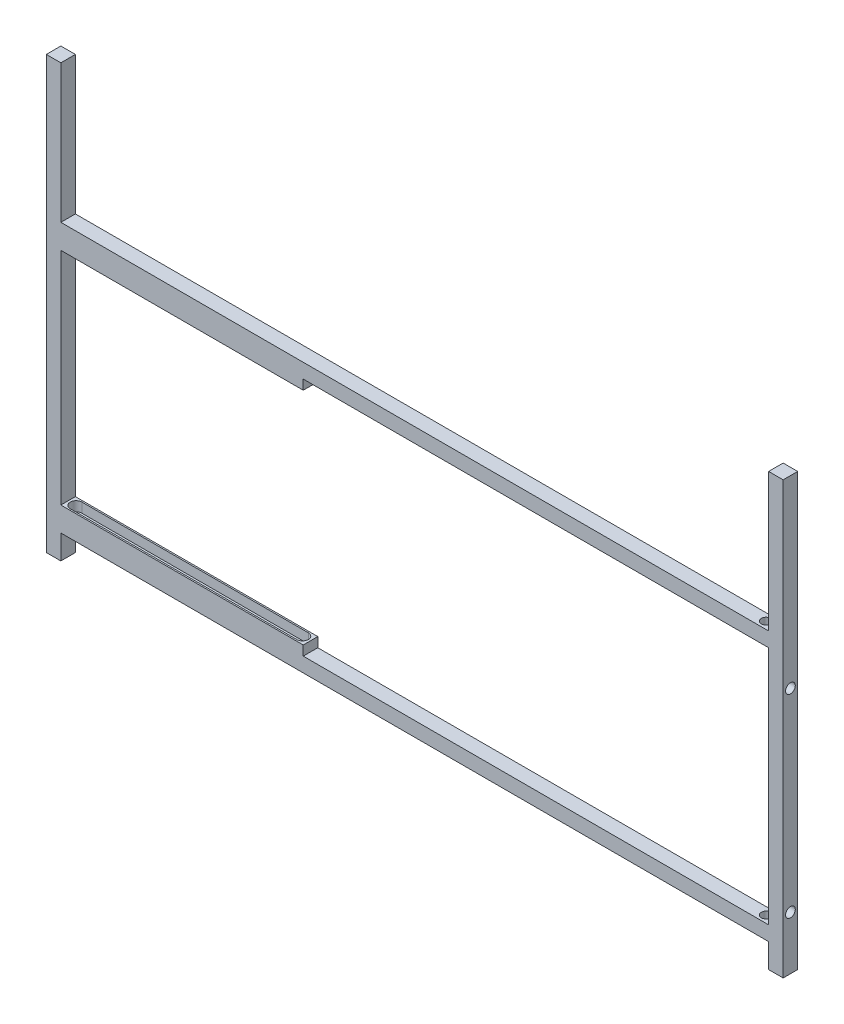
SolidWorks part; units mm, degrees
ref_plane "Front Plane" through (0, 0, 0) normal (0, 0, 1) x (1, 0, 0)
ref_plane "Top Plane" through (0, 0, 0) normal (0, 1, 0) x (1, 0, 0)
ref_plane "Right Plane" through (0, 0, 0) normal (1, 0, 0) x (0, 0, -1)
other "Configuration Table"
sketch "Sketch1" plane through (0, 0, 0) normal (0, 1, 0) x (1, 0, 0)
  line L8 (0, 0) -> (0, 55.1158) construction
  line L9 (-7.5, 7.5) -> (7.5, 7.5)
  line L10 (-7.5, 7.5) -> (-7.5, -7.5)
  line L11 (-7.5, -7.5) -> (7.5, -7.5)
  line L12 (7.5, 7.5) -> (7.5, -7.5)
  line L13 (-7.5, 7.5) -> (7.5, -7.5) construction
  line L14 (-7.5, -7.5) -> (7.5, 7.5) construction
  line L15 (372.5, 47.674) -> (372.5, -59.4029) construction
  line L16 (752.5, -7.5) -> (737.5, -7.5)
  line L17 (737.5, 7.5) -> (737.5, -7.5)
  line L18 (752.5, 7.5) -> (737.5, 7.5)
  line L19 (752.5, 7.5) -> (752.5, -7.5)
  point P0 (0, 0)
  dimension "D1" = 15
  dimension "D2" = 15
  dimension "D3" = 372.5
extrude "Boss-Extrude1" add sketch "Sketch1" against normal blind 445
sketch "Sketch2" plane through (7.5, 0, 0) normal (1, 0, 0) x (0, 0, -1)
  line L0 (7.5, -445) -> (7.5, 0) construction
  line L1 (-7.5, -405) -> (7.5, -405)
  line L2 (-7.5, -405) -> (-7.5, -420)
  line L3 (-7.5, -420) -> (7.5, -420)
  line L4 (7.5, -405) -> (7.5, -420)
  line L5 (-7.5, -405) -> (7.5, -420) construction
  line L6 (-7.5, -420) -> (7.5, -405) construction
  line L7 (-7.5, -445) -> (7.5, -445) construction
  line L8 (-7.5, -445) -> (-7.5, 0) construction
  line L9 (-7.5, -142.5) -> (7.5, -142.5)
  line L10 (-7.5, -142.5) -> (-7.5, -157.5)
  line L11 (-7.5, -157.5) -> (7.5, -157.5)
  line L12 (7.5, -142.5) -> (7.5, -157.5)
  line L13 (-7.5, -142.5) -> (7.5, -157.5) construction
  line L14 (-7.5, -157.5) -> (7.5, -142.5) construction
  point P0 (0, -412.5)
  point P9 (0, -150)
  dimension "D1" = 15
  dimension "D2" = 15
  dimension "D3" = 25
  dimension "D4" = 15
  dimension "D5" = 15
  dimension "D6" = 150
extrude "Boss-Extrude2" add sketch "Sketch2" along normal up to surface (730 mm away) up to face at (737.5, -222.5, 0)
sketch "Sketch3" plane through (7.5, 0, 0) normal (1, 0, 0) x (0, 0, -1)
  line L0 (0, 0) -> (0, 101.9802) construction
  circle A0 centre (0, -190) radius 5
  circle A1 centre (0, -390) radius 5
  dimension "D1" = 10
  dimension "D2" = 10
  dimension "D3" = 200
  dimension "D4" = 190
extrude "Cut-Extrude1" cut sketch "Sketch3" along normal blind 900
sketch "Sketch4" plane through (0, -405, 0) normal (0, 1, 0) x (1, 0, 0)
  line L0 (737.5, -7.5) -> (7.5, -7.5) construction
  line L1 (7.5, 7.5) -> (257.5, 7.5)
  line L2 (7.5, 7.5) -> (7.5, -7.5)
  line L3 (7.5, -7.5) -> (257.5, -7.5)
  line L4 (257.5, 7.5) -> (257.5, -7.5)
  line L5 (7.5, 7.5) -> (257.5, -7.5) construction
  line L6 (7.5, -7.5) -> (257.5, 7.5) construction
  line L7 (7.5, 7.5) -> (7.5, -7.5) construction
  line L8 (7.5, -7.5) -> (7.5, 7.5) construction
  line L9 (737.5, 7.5) -> (7.5, 7.5) construction
  line L10 (15.7, 0) -> (249.3, 0) construction
  line L11 (15.7, 6) -> (249.3, 6)
  line L12 (15.7, -6) -> (249.3, -6)
  arc A0 (15.7, 6) -> (15.7, -6) centre (15.7, 0) ccw
  arc A1 (249.3, -6) -> (249.3, 6) centre (249.3, 0) ccw
  point P0 (132.5, 0)
  point P9 (132.5, 0)
  line M3 (7.5, -7.5) -> (737.5, -7.5)
  line M5 (737.5, 7.5) -> (7.5, 7.5)
  line M6 (7.5, 7.5) -> (7.5, -7.5)
  dimension "D4" = 6
  dimension "D1" = 250
  dimension "D2" = 8.2
  dimension "D3" = 1.5
  dimension "D5" = 12
extrude "Boss-Extrude5" add sketch "Sketch4" along normal blind 10 contours L4 A1 L12 A0 L11 M5 M6 M3
sketch "Sketch6" plane through (0, -157.5, 0) normal (0, -1, 0) x (1, 0, 0)
  line L0 (7.5, -7.5) -> (257.5, -7.5) construction
  line L1 (7.5, -7.5) -> (7.5, 7.5) construction
  line L2 (7.5, 7.5) -> (257.5, 7.5) construction
  line L3 (257.5, -7.5) -> (257.5, 7.5) construction
  line L7 (15.7, 6) -> (249.3, 6) construction
  line L8 (15.7, -6) -> (249.3, -6) construction
  line L9 (7.5, -7.5) -> (257.5, -7.5)
  line L10 (7.5, -7.5) -> (7.5, 7.5)
  line L11 (7.5, 7.5) -> (257.5, 7.5)
  line L12 (257.5, -7.5) -> (257.5, 7.5)
  line L16 (15.7, 6) -> (249.3, 6)
  line L17 (15.7, -6) -> (249.3, -6)
  arc A0 (249.3, -6) -> (249.3, 6) centre (249.3, 0) ccw construction
  arc A1 (15.7, 6) -> (15.7, -6) centre (15.7, 0) ccw construction
  arc A2 (249.3, -6) -> (249.3, 6) centre (249.3, 0) ccw
  arc A3 (15.7, 6) -> (15.7, -6) centre (15.7, 0) ccw
  line M1 (7.5, -7.5) -> (737.5, -7.5)
  line M3 (737.5, 7.5) -> (7.5, 7.5)
  line M4 (7.5, 7.5) -> (7.5, -7.5)
extrude "Boss-Extrude6" add sketch "Sketch6" along normal blind 10 contours L12 A3 L16 A2 L17 M1 M3 M4
sketch "Sketch7" plane through (0, -142.5, 0) normal (0, 1, 0) x (1, 0, 0)
  line L0 (752.5, -7.5) -> (752.5, 7.5) construction
  line L1 (737.5, 7.5) -> (7.5, 7.5) construction
  circle A0 centre (727.5, 0) radius 5
  dimension "D1" = 10
  dimension "D2" = 25
  dimension "D3" = 7.5
extrude "Cut-Extrude2" cut sketch "Sketch7" against normal blind 500
